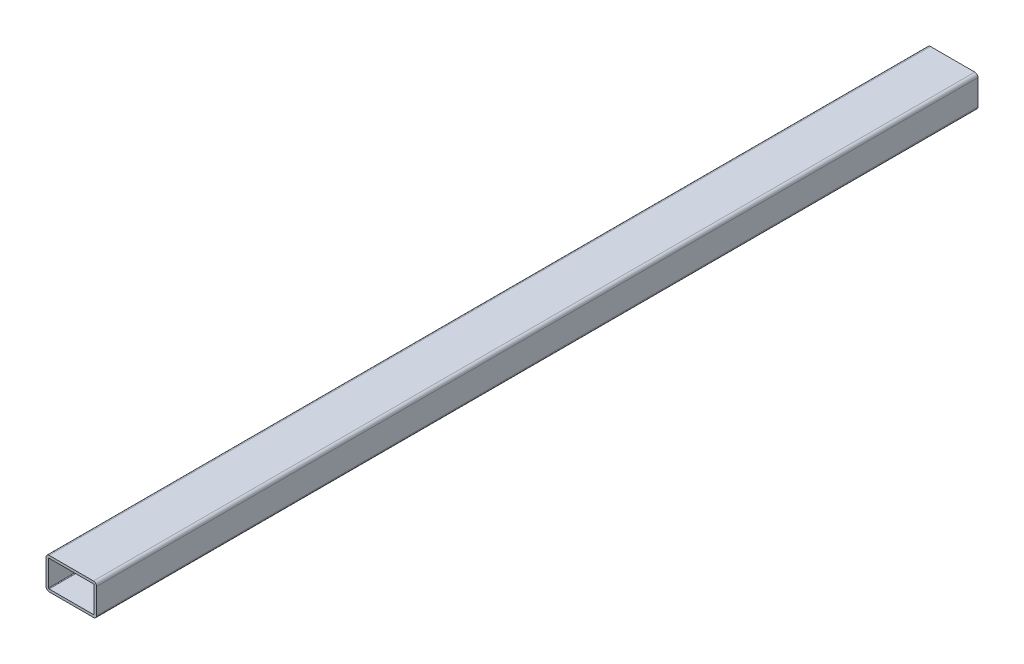
SolidWorks part; units mm, degrees
material "1023 Carbon Steel Plate (SS)"
ref_plane "Front Plane" through (0, 0, 0) normal (0, 0, 1) x (1, 0, 0)
ref_plane "Top Plane" through (0, 0, 0) normal (0, 1, 0) x (1, 0, 0)
ref_plane "Right Plane" through (0, 0, 0) normal (1, 0, 0) x (0, 0, -1)
sketch "Sketch1" plane through (0, 0, 0) normal (0, 0, 1) x (1, 0, 0)
  line L1 (35, 25) -> (-35, 25)
  line L2 (40, 20) -> (40, -20)
  line L3 (35, -25) -> (-35, -25)
  line L4 (-40, 20) -> (-40, -20)
  line L5 (40, 25) -> (-40, -25) construction
  line L6 (40, -25) -> (-40, 25) construction
  arc A0 (-35, -25) -> (-40, -20) centre (-35, -20) cw
  arc A1 (40, -20) -> (35, -25) centre (35, -20) cw
  arc A2 (35, 25) -> (40, 20) centre (35, 20) cw
  arc A3 (-35, 25) -> (-40, 20) centre (-35, 20) ccw
  point P0 (0, 0)
  dimension "D3" = 5
  dimension "D1" = 80
  dimension "D2" = 50
extrude "Boss-Extrude1" add sketch "Sketch1" along normal blind 1393 contours L4 A0 L3 A1 L2 A2 L1 A3
shell "Shell1" thickness 4
